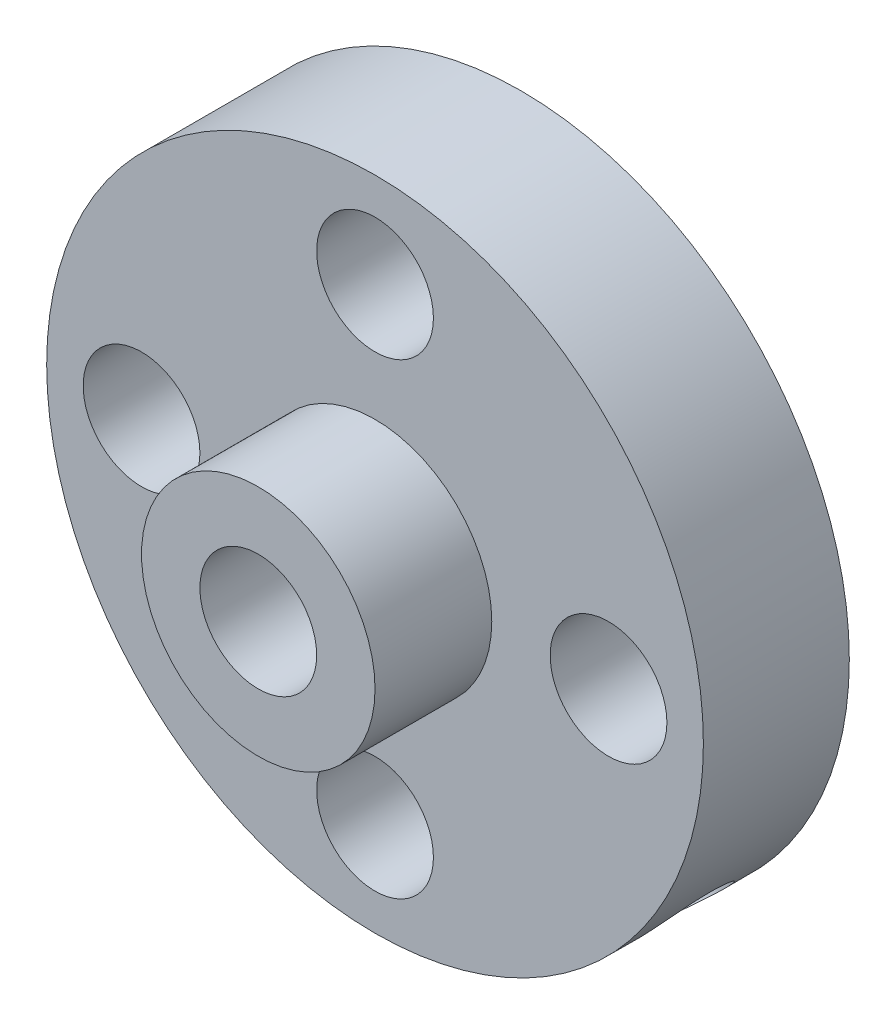
SolidWorks part; units mm, degrees
ref_plane "Front Plane" through (0, 0, 0) normal (0, 0, 1) x (1, 0, 0)
ref_plane "Top Plane" through (0, 0, 0) normal (0, 1, 0) x (1, 0, 0)
ref_plane "Right Plane" through (0, 0, 0) normal (1, 0, 0) x (0, 0, -1)
sketch "Sketch1" plane through (0, 0, 0) normal (0, 0, 1) x (1, 0, 0)
  line L0 (0, 6) -> (0, 0)
  line L1 (0, 11.25) -> (0, 10)
  circle A0 centre (0, 0) radius 11.25
  circle A1 centre (0, 8) radius 2
  circle A2 centre (8, 0) radius 2
  circle A3 centre (0, -8) radius 2
  circle A4 centre (-8, 0) radius 2
  circle A5 centre (0, 0) radius 2
  point P17 (0, 0)
  dimension "D1" = 22.5
  dimension "D3" = 4
  dimension "D4" = 4
  dimension "D2" = 8
extrude "Boss-Extrude1" add sketch "Sketch1" along normal blind 5
sketch "Sketch2" plane through (0, 0, 5) normal (0, 0, 1) x (1, 0, 0)
  circle A0 centre (0, 0) radius 2
  circle A1 centre (0, 0) radius 4
  dimension "D1" = 8
extrude "Boss-Extrude2" add sketch "Sketch2" along normal blind 4
sketch "Sketch3" plane through (0, 0, 5) normal (0, 0, 1) x (1, 0, 0)
  line L0 (0, 0) -> (7.7995, -7.7995)
ref_plane "Plane1" through (7.955, -7.955, 0) normal (0.7071, -0.7071, 0) x (-0.7071, -0.7071, 0)
sketch "Sketch4" plane through (7.955, -7.955, 0) normal (0.7071, -0.7071, 0) x (-0.7071, -0.7071, 0)
  line L0 (0, 0) -> (0, -4.9167)
  circle A0 centre (0, -2.4583) radius 1.5
  dimension "D1" = 3
extrude "Cut-Extrude1" cut sketch "Sketch4" against normal blind 10 contours L0 A0 | L0 A0
